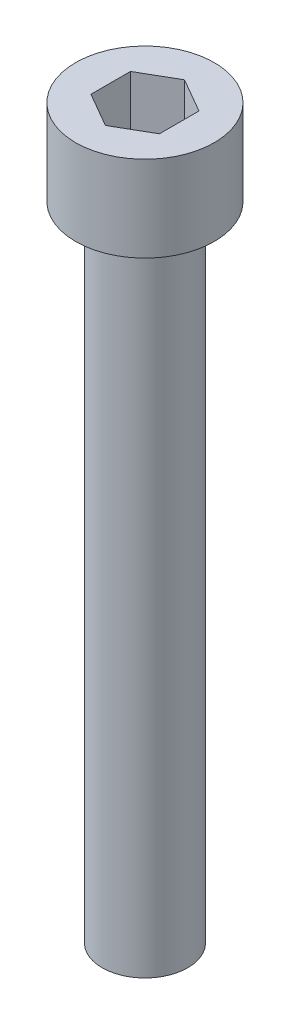
from build123d import *

# Parameters (mm, degrees)
CUT_EXTRUDE_1_DEPTH = 6


with BuildPart() as part:
    # Sketch 1 → Revolve 1 (revolve)
    with BuildSketch(Plane.XY, mode=Mode.PRIVATE) as revolve_1_sk:
        Polygon((0, 10), (-8.1, 10), (-8.1, 0), (-5, 0), (-5, -75), (0, -75), align=None)
    revolve(revolve_1_sk.sketch.rotate(Axis((0, 11.322033898, 0), (0, -1, 0)), 270), axis=Axis((0, 11.322033898, 0), (0, -1, 0)))

    # Sketch 2 → Cut-Extrude 1 (cut)
    with BuildSketch(Plane(origin=(0, 10, 0), x_dir=(1, 0, 0), z_dir=(0, 1, 0))):
        Polygon((0, 4.618802154), (-4, 2.309401077), (-4, -2.309401077), (0, -4.618802154), (4, -2.309401077), (4, 2.309401077), align=None)
    extrude(amount=-CUT_EXTRUDE_1_DEPTH, mode=Mode.SUBTRACT)


solid = part.part
